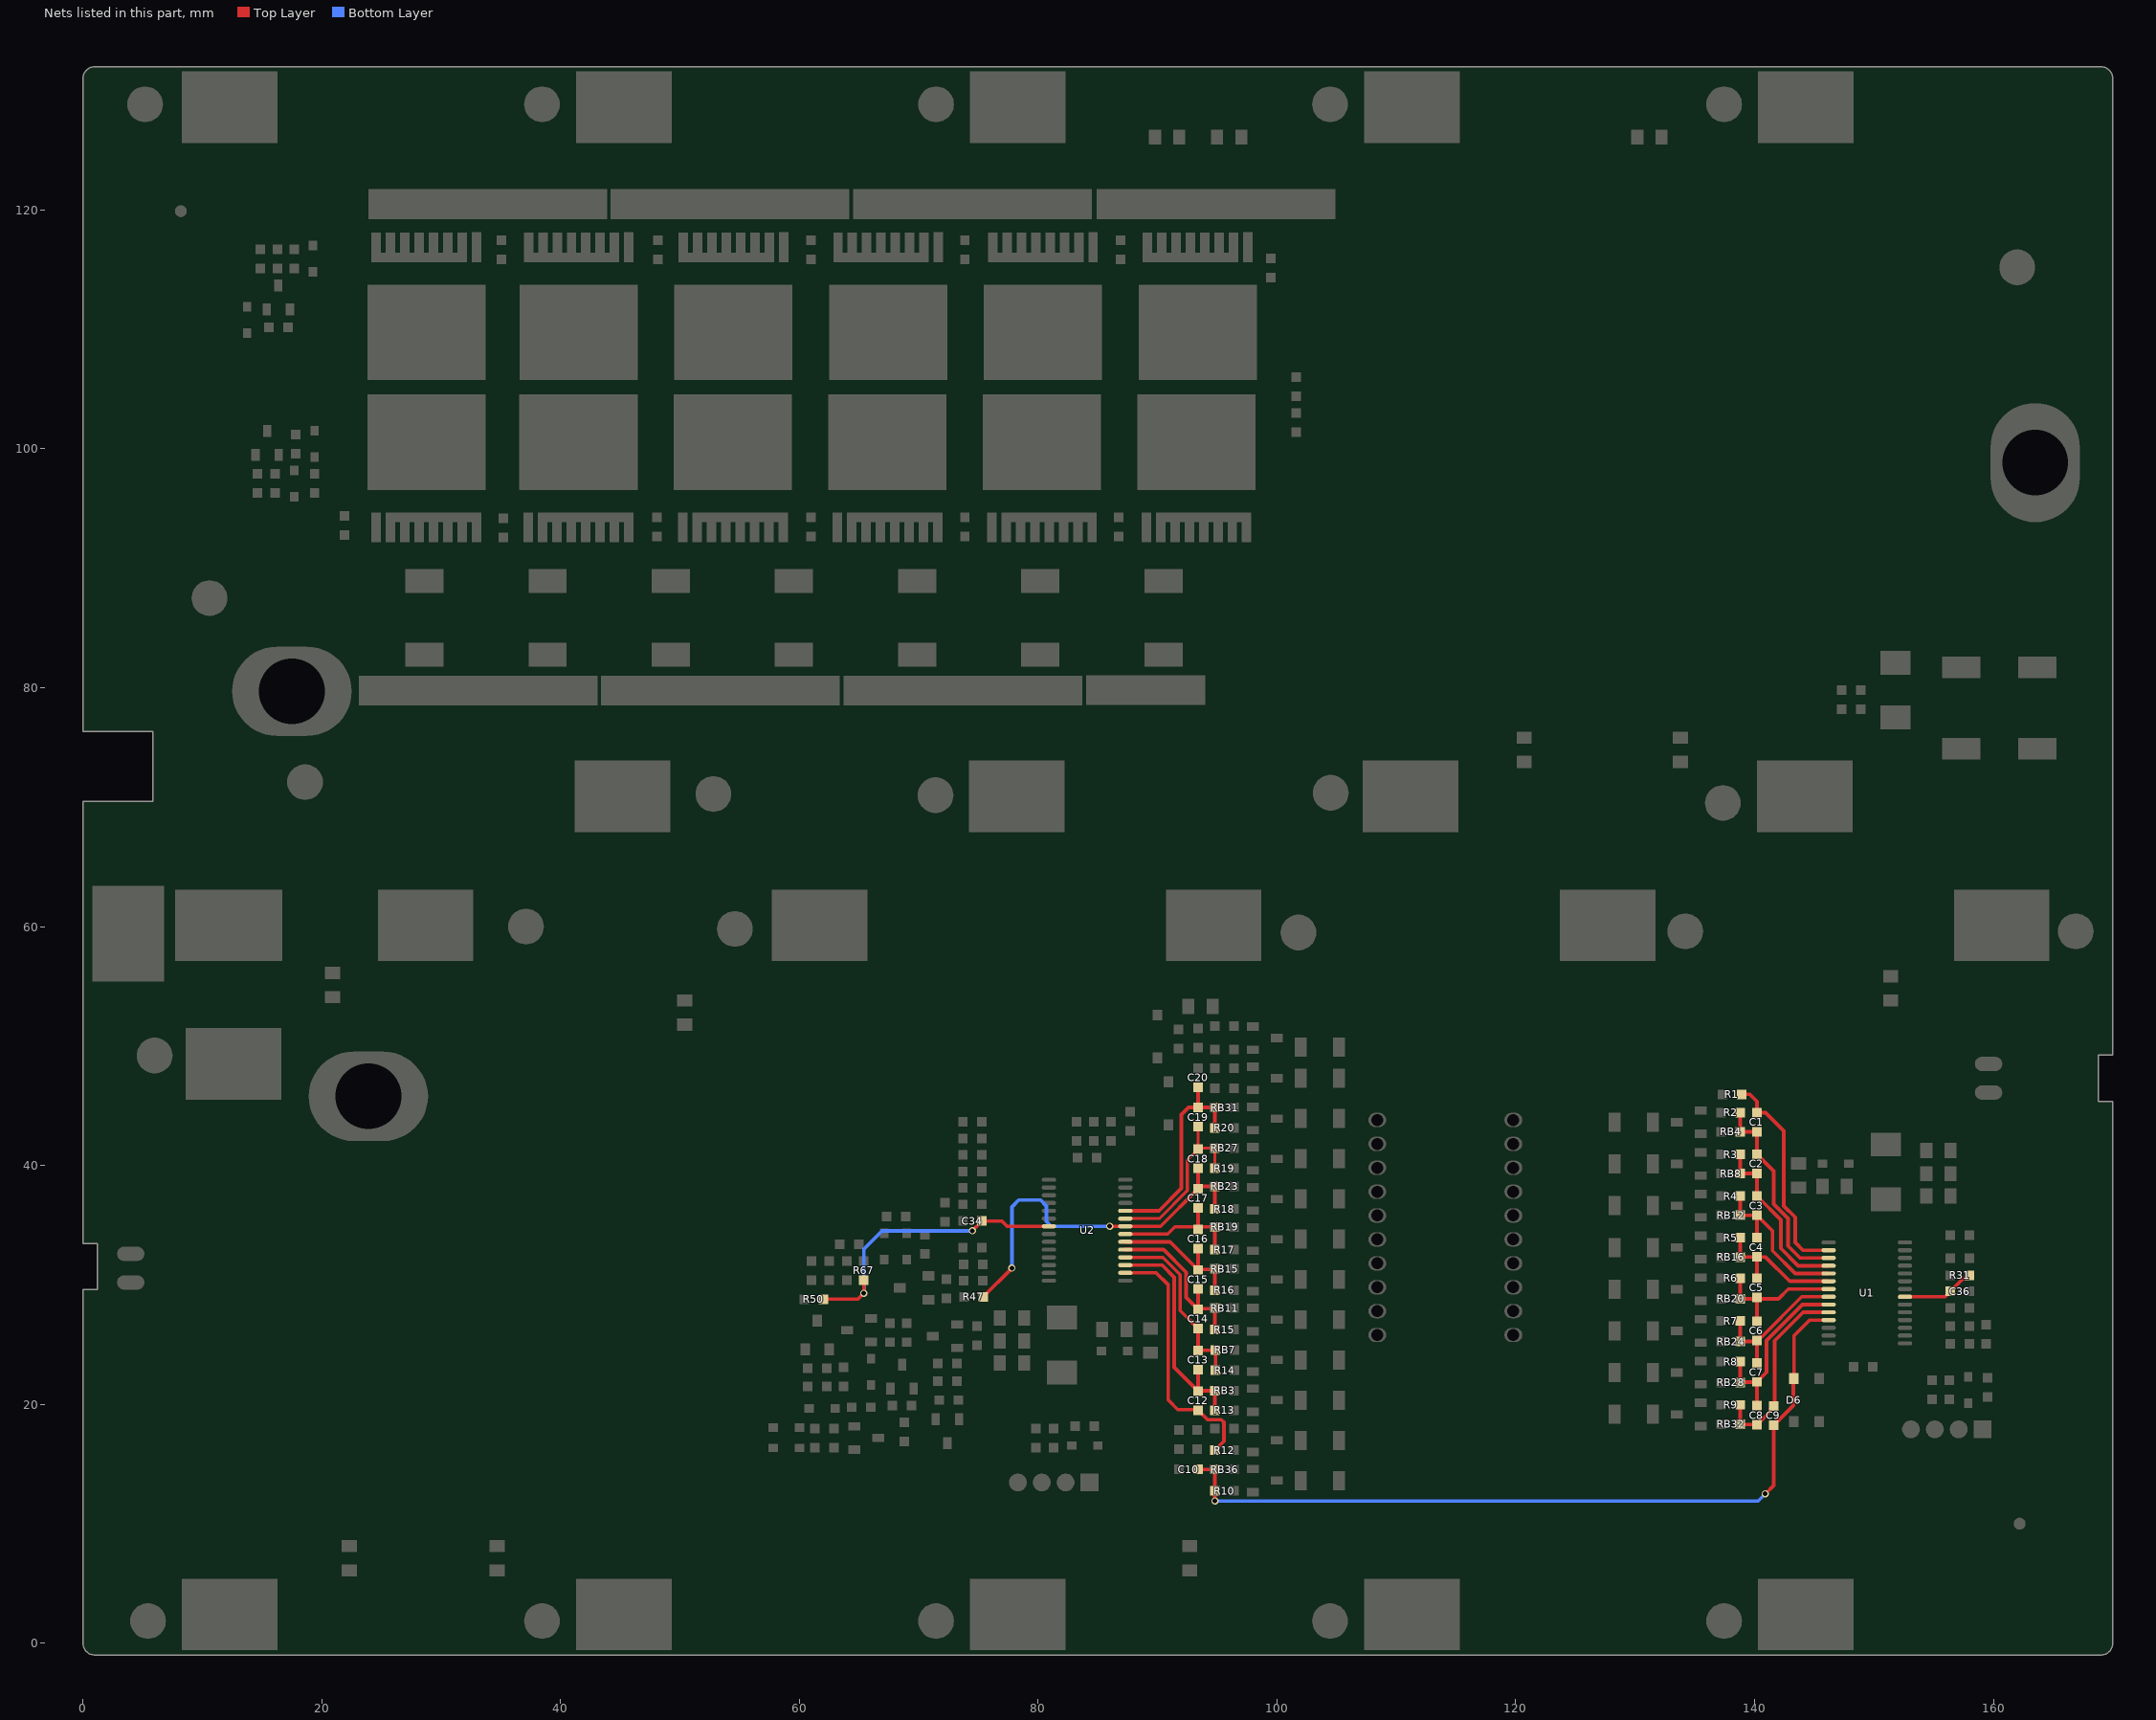
[diagram p0: the nets of this part, all layers, seen from the top]
# Altium PCB MISC82749.PcbDoc (part 4 of 4)
Units mm, origin at the board's own origin, x right, y up, seen from the top; angles counter-clockwise.
Board outline 170 x 133 mm, 2 copper layers (Top Layer, Bottom Layer); 262 components, 170 nets, 783 pads, 1052 vias.

## Via types
v1: diameter 0.7, hole 0.5, Top Layer to Bottom Layer, tented both sides, 953 vias
v2: diameter 0.6, hole 0.4, Top Layer to Bottom Layer, tented both sides, 99 vias

## Nets (pads, with @x,y where several pads share a name; then routed paths per layer and width w, separated by ;. In a path a pad name is that pad's centre, name@x,y a point inside that pad or via, vN(x,y) a via of type N, cw(c..) or ccw(c..) an arc to the next point about the centre after c; other vN are vias at no path point) (continued)
"VC1 S": C9.1 C10.2 D6.1 R10.2 RB36.2 U1.11 | length 68.1
  Top Layer w0.3: C10.2@93.4,14.55 93.45,14.5 93.5,14.55 RB36.2@94.8,14.55 v2(94.8,11.9) ; v2(140.9,12.5) 141.6,13.2 C9.1@141.6,18.25 143.25,19.9 143.25,22.1 D6.1@143.3,22.15 143.3,25.75 144.6,27.05 U1.11@146.2,27.05
  Bottom Layer w0.3: v2(94.8,11.9) 140.3,11.9 v2(140.9,12.5)
"VC2 M": C19.1 C20.2 R20.2 RB31.2 U2.10 | length 18.1
  Top Layer w0.3: U2.10@87.3,36.2 90.125,36.2 92,38.075 92,44.25 92.6,44.85 C19.1@93.4,44.85 ; C20.2@93.4,46.55 C19.1@93.4,44.85 ; R20.2@94.8,43.15 RB31.2@94.8,44.85 C19.1@93.4,44.85
"VC2 S": C8.1 C9.2 R9.2 RB32.2 U1.10 | length 16.2
  Top Layer w0.3: R9.2@138.8,19.882 RB32.2@138.8,18.332 138.825,18.307 140.175,18.307 C8.1@140.2,18.282 141.35,19.432 141.35,19.6 C9.2@141.6,19.85 ; C9.2@141.684,19.766 141.684,25.32 144.064,27.7 U1.10@146.2,27.7
"VC3 M": C18.1 C19.2 R19.2 RB27.2 U2.9 | length 15
  Top Layer w0.254: U2.9@87.3,35.55 90.15,35.55 92.5,37.9 92.5,40.45 C18.1@93.4,41.35 C18.1@93.4,41.45 ; C19.2@93.4,43.25 C18.1@93.4,41.45 ; R19.2@94.8,39.75 RB27.2@94.8,41.45 C18.1@93.4,41.45
"VC3 S": C7.1 C8.2 R8.2 RB28.2 U1.9 | length 15.4
  Top Layer w0.3: R8.2@138.8,23.573 RB28.2@138.8,21.83 138.821,21.852 140.179,21.852 C7.1@140.2,21.873 ; C8.2@140.2,19.883 C7.1@140.2,21.873 ; U1.9@146.2,28.35 144.007,28.35 141,25.343 141,22.673 C7.1@140.2,21.873
"VC4 M": C17.1 C18.2 R18.2 R47.2 RB23.2 U2.8 | length 32.1
  Top Layer w0.3: R47.2@75.4,29 v2(77.8,31.4) ; v2(86,34.9) U2.8@87.3,34.9 90.25,34.9 C17.1@93.4,38.05 ; C18.2@93.4,39.75 93.4,38.25 RB23.2@94.8,38.25 R18.2@94.8,36.35
  Bottom Layer w0.3: v2(77.8,31.4) 77.8,36.52 78.38,37.1 80.2,37.1 80.7,36.6 80.7,35.3 81.1,34.9 v2(86,34.9)
"VC4 S": C6.1 C7.2 R7.2 RB24.2 U1.8 | length 12.6
  Top Layer w0.3: R7.2@138.8,26.964 RB24.2@138.8,25.25 C6.1@140.2,25.25 ; C7.2@140.2,23.473 C6.1@140.2,25.25 ; U1.8@146.2,29 143.95,29 140.55,25.6 140.45,25.6 C6.1@140.2,25.35 ; C6.1@140.2,25.25 C6.1@140.2,25.35 ; C6.1@140.2,25.25 C6.1@140.2,25.35
"VC5 M": C16.1 C17.2 R17.2 RB19.2 U2.7 | length 11.4
  Top Layer w0.3: U2.7@87.3,34.25 90.849,34.25 91.449,34.85 C16.1@93.4,34.85 ; C16.1@93.4,34.65 C16.1@93.4,34.85 ; C17.2@93.4,36.45 C16.1@93.4,34.85 ; R17.2@94.8,32.95 RB19.2@94.8,34.85 C16.1@93.4,34.85
"VC5 S": C5.1 C6.2 R6.2 RB20.2 U1.7 | length 11.5
  Top Layer w0.3: R6.2@138.8,30.555 RB20.2@138.8,28.826 C5.1@140.2,28.826 ; C6.2@140.2,26.95 C5.1@140.2,28.826 ; C5.1@140.2,28.955 C5.1@140.2,28.826 ; U1.7@146.2,29.65 142.818,29.65 141.994,28.826 C5.1@140.2,28.826
"VC6 M": C15.1 C16.2 R16.2 RB15.2 U2.6 | length 12.1
  Top Layer w0.3: U2.6@87.3,33.6 91.05,33.6 C15.1@93.4,31.25 ; C16.2@93.4,33.05 C15.1@93.4,31.25 ; R16.2@94.8,29.55 RB15.2@94.8,31.35 94.75,31.3 93.45,31.3 C15.1@93.4,31.25
"VC6 S": C4.1 C5.2 R5.2 RB16.2 U1.6 | length 11.7
  Top Layer w0.3: R5.2@138.8,33.945 RB16.2@138.8,32.324 C4.1@140.2,32.324 ; C5.2@140.2,30.555 C4.1@140.2,32.324 ; C4.1@140.2,32.345 C4.1@140.2,32.324 ; U1.6@146.2,30.3 142.95,30.3 140.926,32.324 C4.1@140.2,32.324
"VC7 M": C14.1 C15.2 R15.2 RB11.2 U2.5 | length 14.3
  Top Layer w0.3: U2.5@87.3,32.95 90.5,32.95 92.4,31.05 92.4,28.95 C14.1@93.4,27.95 ; C15.2@93.4,29.65 C14.1@93.4,27.95 ; R15.2@94.8,26.25 RB11.2@94.8,28.05 94.75,28 93.45,28 C14.1@93.4,27.95
"VC7 S": C3.1 C4.2 R4.2 RB12.2 U1.5 | length 13.9
  Top Layer w0.3: R4.2@138.8,37.436 RB12.2@138.8,35.822 C3.1@140.2,35.822 ; C4.2@140.2,33.945 C3.1@140.2,35.822 ; C3.1@140.2,35.836 C3.1@140.2,35.822 ; U1.5@146.2,30.95 143.4,30.95 141.5,32.85 141.5,34.522 140.45,35.572 140.45,35.586 140.214,35.822 C3.1@140.2,35.822
"VC8 M": C13.1 C14.2 R14.2 RB7.2 U2.4 | length 15.3
  Top Layer w0.3: U2.4@87.3,32.3 90.443,32.3 91.9,30.843 91.9,27.85 C14.2@93.4,26.35 C13.1@93.4,24.5 93.425,24.525 94.825,24.525 RB7.2@94.85,24.55 R14.2@94.85,22.85
"VC8 S": C2.1 C3.2 R3.2 RB8.2 U1.4 | length 14.6
  Top Layer w0.3: R3.2@138.8,40.927 RB8.2@138.8,39.32 138.804,39.323 140.196,39.323 C2.1@140.2,39.327 C3.2@140.2,37.436 ; C3.2@140.3,37.337 142.2,35.436 142.2,33.05 143.65,31.6 U1.4@146.2,31.6
"VC9 M": C12.1 C13.2 R13.2 RB3.2 U2.3 | length 19.8
  Top Layer w0.3: U2.3@87.3,31.65 90.386,31.65 91.4,30.636 91.4,23.1 C12.1@93.4,21.1 ; C13.2@93.4,22.9 C12.1@93.4,21.1 ; R13.2@94.8,19.5 RB3.2@94.8,21.15 94.775,21.125 93.425,21.125 C12.1@93.4,21.1
"VC9 S": C1.1 C2.2 R2.2 RB4.2 U1.3 | length 17.5
  Top Layer w0.3: R2.2@138.8,44.418 RB4.2@138.8,42.818 C1.1@140.2,42.818 C2.2@140.2,40.927 141.6,39.527 141.6,36.75 142.8,35.55 142.8,33.25 143.8,32.25 U1.3@146.2,32.25
"VC10 M": C12.2 R12.2 U2.2 | length 21.7
  Top Layer w0.3: U2.2@87.3,31 89.893,31 90.9,29.993 90.9,20.35 91.7,19.55 93.35,19.55 C12.2@93.4,19.5 94.2,18.7 95.345,18.7 95.55,18.495 95.55,16.9 R12.2@94.8,16.15
"VC10 S": C1.2 R1.2 U1.2 | length 18.2
  Top Layer w0.3: R1.2@138.9,45.95 139.6,45.95 140.2,45.35 C1.2@140.2,44.418 140.932,44.418 142.454,42.896 142.454,36.604 143.4,35.657 143.4,33.55 144.05,32.9 U1.2@146.2,32.9
VCC_M: C34.2 R50.2 R67.2 U2.21 | length 25.1
  Top Layer w0.3: R50.2@62,28.8 64.9,28.8 v2(65.4,29.3) R67.2@65.4,30.4 ; v2(74.49,34.52) 74.49,34.53 C34.2@75.3,35.34 76.96,35.34 77.4,34.9 U2.21@80.9,34.9
  Bottom Layer w0.3: v2(65.4,29.3) 65.4,33 66.92,34.52 v2(74.49,34.52)
VCC_S: C36.2 R31.1 U1.21 | length 6.1
  Top Layer w0.3: U1.21@152.6,29 155.95,29 157.5,30.55 157.75,30.55 R31.1@158,30.8
pads on no net: U1.1 U1.27 U2.1 U2.27

## Polygon pours and split planes (outlines as drawn)
NetR68_2 on Top Layer "NONET_L02_P-001" (solid, remove dead copper, pour order 188): 155.6,50.4 161.1,50.4 161.4,50.1 161.4,47.5 155.7,47.5 155.6,47.6
NetR67_1 on Top Layer "NONET_L02_P-001" (solid, remove dead copper, pour order 187): 155.6,47 155.6,44.2 161.1,44.2 161.1,47
P-/C- on Top Layer "NONET_L02_P-001" (solid, remove dead copper, pour order 121): 20.8,124 127.5,124 127.75,123.75 128.7,122.8 170,122.8 170,79 170.1,78.9 102.6,78.9 102.6,105.2 102.4,105.4 101.1,105.4 101.1,116.3 100.831,116.569 99.431,116.569 99.062,116.938 99.062,118.338 96.96,118.338 96.96,115.689 96.821,115.55 87.65,115.55 87.5,115.7 87.5,118.1 87.262,118.338 84,118.338 84,115.55 74.46,115.55 74.46,118.25 74.372,118.338 71.04,118.338 71.04,115.55 61.56,115.55 61.56,118.25 61.472,118.338 58.08,118.338 58.08,115.55 48.76,115.55 48.76,118.35 45.132,118.35 45.12,118.338 45.12,115.55 35.66,115.55 35.66,118.05 35.372,118.338 32.36,118.338 32.36,115.61 32.3,115.55 20.402,115.55 19.8,116.152 19.8,123
B4 on Top Layer "NONET_L02_P-001" (solid, remove dead copper, pour order 139): 86.65,67.55 89.5,70.4 89.5,74.6 68.3,74.6 68.2,74.5 68.2,70.1 70.75,67.55
B14 on Top Layer "NONET_L02_P-001" (solid, remove dead copper, pour order 138): 98.3,63.4 98.9,62.8 105.5,62.8 105.8,62.5 105.8,59.375 105.8,55.35 88,55.35 88,63.4
B13 on Top Layer "NONET_L02_P-001" (solid, remove dead copper, pour order 131): 100,7.15 126.15,7.15 126.9,6.4 126.9,-0.4 126.4,-0.9 109.4,-0.9 100,-0.9
B+ on Top Layer "NONET_L02_P-001" (solid, remove dead copper, pour order 179): 0.1,27.546 30.993,27.546 31.5,27.039 31.5,9.6 31,9.1 0.6,9.1 0.1,9.6
B17 on Top Layer "NONET_L02_P-001" (solid, remove dead copper, pour order 129): 61.15,7.15 61.5,6.8 61.5,-0.9 34,-0.9 34,7.15
B+ on Top Layer "NONET_L02_P-001" (solid, remove dead copper, pour order 178): 155.1,44.2 155.1,52.7 125.2,52.7 125.2,43.1 125.5,42.8 129.9,42.8 129.9,44.8 131.6,46.5 141.5,46.5 144.8,44.2
B10 on Top Layer "NONET_L02_P-001" (solid, remove dead copper, pour order 170): 162.1,15.2 161.5,14.6 153.7,14.6 153.5,14.8 153.5,20.75 153.15,21.1 144.227,21.1 143.607,20.48 143.607,19.752 141.957,18.102 141.957,8.743 142.3,8.4 169.9,8.4 170,8.5 170,35.6 170,57.4 162.1,57.4
GND on Top Layer "NONET_L02_P-001" (solid, remove dead copper, pour order 186): 85.7,51 85.4,51.3 74,51.3 72.2,49.5 72.2,45.4 72.3,45 85.1,45 85.7,45.6
B12 on Top Layer "NONET_L02_P-001" (solid, remove dead copper, pour order 141): 120.9,62.6 121.2,62.9 125.5,62.9 141.7,62.9 141.7,55.35 120.9,55.35
NetC33_1 on Top Layer "NONET_L02_P-001" (solid, remove dead copper, pour order 184): 9.2,34.9 9.1,35 0.4,35 0.25,34.85 0.25,31.7 9.2,31.7
GND on Top Layer "NONET_L02_P-001" (solid, remove dead copper, pour order 183): 0.3,31.3 9.3,31.3 9.3,29.55 9.3,28.3 9.2,28.2 0.5,28.2 0.3,28.4
GND on Top Layer "NONET_L02_P-001" (solid, remove dead copper, pour order 182): 68.6,40.4 68.9,40.7 68.9,49.3 67.7,50.5 54.7,50.5 36.1,50.384 36.1,40.4
B10 on Top Layer "NONET_L02_P-001" (solid, remove dead copper, pour order 177): 116.1,78.2 116.1,76.1 144.8,76.1 144.8,78.3 116.5,78.3
VBAT_S on Top Layer "NONET_L02_P-001" (solid, remove dead copper, pour order 168): 154.1,34.3 154.1,33.8 154.2,33.7 154.7,33.7 155.712,34.712 157.12,36.12 157.12,42.98 156.8,43.3 155.7,43.3 155.7,35.9
B10 on Top Layer "NONET_L02_P-001" (solid, remove dead copper, pour order 167): 155.05,36.45 155.05,36.15 153.7,34.8 147.6,34.8 147.2,35.2 147.2,39.1 152.2,39.1 153.225,40.125 155.075,40.125 155.1,40.1 155.1,36.5
NetD1_1 on Top Layer "NONET_L02_P-001" (solid, remove dead copper, pour order 166): 152.9,40.5 154.9,40.5 155.1,40.7 155.1,43.4 147.2,43.4 147.2,39.5 151.9,39.5
NetC23_2 on Top Layer "NONET_L02_P-001" (solid, remove dead copper, pour order 165): 142.875,39.15 142.875,37.125 143.6,36.4 146.2,36.4 146.2,40.8 146.1,40.9 145.2,40.9 144.8,40.5 144.8,39.425 144.475,39.1 143.1,39.1
B6 on Top Layer "NONET_L02_P-001" (solid, remove dead copper, pour order 140): 121.8,68.5 121.6,68.3 115.2,68.3 114.7,67.8 103.151,67.8 102.5,68.451 102.5,73.7 103.2,74.4 121.4,74.4 121.8,74
VBAT_M on Top Layer "NONET_L02_P-001" (solid, remove dead copper, pour order 164): 77.7,27.824 80.376,30.5 78.805,30.5 76.09,27.785 76.09,21.61 76.5,21.2 77.5,21.2 77.7,21.4
NetC24_2 on Top Layer "NONET_L02_P-001" (solid, remove dead copper, pour order 162): 88.3,25.1 88.7,25.5 90.1,25.5 90.2,25.6 90.2,27.016 90.235,27.051 86.8,27 86.8,23.6 88.3,23.6
GND on Top Layer "NONET_L02_P-001" (solid, remove dead copper, pour order 161): 86.2,25.7 86.2,27.2 86.3,27.3 90.2,27.3 90.2,29.2 89.702,29.698 86.102,29.698 85.5,30.3 85.5,38.4 82.8,38.4 82,37.6 82,29.8 81.6,29.4 79.7,29.4 78.3,28 78.3,24.6 78.4,24.5 80.3,24.5 81.3,25.5 86,25.5
NetD2_1 on Top Layer "NONET_L02_P-001" (solid, remove dead copper, pour order 160): 78.4,24.2 78.4,22.2 79.5,21.1 85.7,21.1 85.9,21.3 85.9,24.9 81.7,24.9 81,24.2 78.7,24.2
GND on Top Layer "NONET_L02_P-001" (solid, remove dead copper, pour order 101): 95.1,75.9 40.6,75.9 38.8,74.1 38.8,67.9 5.85,67.9 5.85,76.35 0,76.35 0,114.5 0.5,115 11.2,115 11.8,114.4 11.8,93 14.9,89.9 23.8,89.9 24.1,89.6 24.1,85.6 26.1,83.6 95.1,83.6 95.9,82.8 95.9,76.7
NetC45_2 on Top Layer "NONET_L02_P-001" (solid, remove dead copper, pour order 117): 98.3,88 102,88 102,94.1 101.5,94.6 89.92,94.6 89.91,94.61 89.91,92.06 89.68,91.83 86.17,91.83 85.95,92.05 85.95,94.12 85.46,94.61 76.97,94.61 76.97,92.15 76.732,91.912 73.288,91.912 73.05,92.15 73.05,94.35 72.7,94.7 64.12,94.7 64.03,94.61 64.03,92.08 63.8,91.85 60.55,91.85 60.35,92.05 60.35,94.55 60.2,94.7 51.18,94.7 51.09,94.61 51.09,91.94 50.85,91.7 47.6,91.7 47.15,92.15 47.15,94.65 47,94.8 38.34,94.8 38.15,94.61 38.15,91.9 37.95,91.7 34.6,91.7 34.35,91.95 34.35,94.15 33.89,94.61 25.21,94.61 25.21,88.19 25.4,88
B+ on Top Layer "NONET_L02_P-001" (solid, remove dead copper, pour order 134): 31.6,36.5 2.7,36.5 0.9,38.3 0.9,63.55 19.3,63.55 19.3,53.9 19.7,53.5 31.4,53.5 31.6,53.3
B9 on Top Layer "NONET_L02_P-001" (solid, remove dead copper, pour order 127): 131.7,131.998 131.7,125.2 170,125.2 170,132.303
B+ on Top Layer "NONET_L02_P-001" (solid, remove dead copper, pour order 144): 150.8,77.7 170.1,77.7 170.1,68.35 150.8,68.35
B8 on Top Layer "NONET_L02_P-001" (solid, remove dead copper, pour order 143): 129.7,74.4 149.2,74.4 149.2,68 129.7,68
B10 on Top Layer "NONET_L02_P-001" (solid, remove dead copper, pour order 142): 147.8,63 169.5,63 169.7,62.8 169.7,55.25 147.8,55.25
B16 on Top Layer "NONET_L02_P-001" (solid, remove dead copper, pour order 137): 49.4,63 52.1,63 52.4,63.3 68.5,63.3 68.5,53.3 49.4,53.3
B2 on Top Layer "NONET_L02_P-001" (solid, remove dead copper, pour order 136): 61.1,68.2 61,68.1 56,68.1 55.55,67.65 40.1,67.65 40.1,73.7 40.9,74.5 61.1,74.5
B18 on Top Layer "NONET_L02_P-001" (solid, remove dead copper, pour order 135): 34.8,63.5 35.3,63 44.4,63 44.4,55.45 20,55.45 20,63.5
B11 on Top Layer "NONET_L02_P-001" (solid, remove dead copper, pour order 133): 169.7,7.15 170.2,6.45 170.2,-0.45 169.75,-0.9 133,-0.9 133,7.15
B15 on Top Layer "NONET_L02_P-001" (solid, remove dead copper, pour order 130): 93.65,7.15 94.3,6.5 94.3,-0.5 93.9,-0.9 76.4,-0.9 67,-0.9 67,7.15
B19 on Top Layer "NONET_L02_P-001" (solid, remove dead copper, pour order 128): 0,6.6 24.1,6.6 24.1,-0.65 23.75,-1 0,-1
B7 on Top Layer "NONET_L02_P-001" (solid, remove dead copper, pour order 126): 96.4,131.979 96.4,125.2 124.7,125.2 124.7,132.205
B5 on Top Layer "NONET_L02_P-001" (solid, remove dead copper, pour order 125): 61.9,131.967 61.9,125.2 90.6,125.2 90.6,132.196
B3 on Top Layer "NONET_L02_P-001" (solid, remove dead copper, pour order 124): 33,132 33,125.2 59.7,125.2 59.7,132.213
B1 on Top Layer "NONET_L02_P-001" (solid, remove dead copper, pour order 123): 30.5,125.4 30.5,132.191 24,132.191 0,132 0,125 18.6,125 19,125.4
MSO_D- on Top Layer "NONET_L02_P-001" (solid, remove dead copper, pour order 106): 22.105,95.995 20.3,97.8 20.3,113.8 21.093,114.593 23.143,114.593 23.15,114.6 98.25,114.6 98.95,113.9 98.95,113.85 100.6,113.85 100.6,95.995
GND on Bottom Layer "NONET_L02_P-001" (solid, remove dead copper, pour order 180): 63.043,29.857 63.043,32.057 62.8,32.3 62,32.3 61.6,32.7 61.6,36.1 62.995,37.495 80.705,37.495 81.2,37 81.2,35.7 81.5,35.4 84.05,35.4 86.4,35.4 86.6,35.2 86.6,34.3 86.4,34.1 80,34.1 79.3,33.4 79.3,22.7 81.2,20.8 87.6,20.8 87.9,21.1 87.9,23.5 88.5,24.1 102.9,24.1 103.3,24.5 103.2,24.6 103.2,43.4 57,43.4 56.869,43.269 35.769,43.269 34.8,42.3 34.8,15.6 37.1,13.3 76.9,13.3 77.6,14 77.6,15.5 77.4,15.7 67.4,15.7 63.1,20 63.1,29.8
B+ on Bottom Layer "NONET_L02_P-001" (solid, remove dead copper, pour order 172): 155.3,11.5 158.6,14.8 158.6,37.2 150.8,45 150.85,76.2 150.95,76.3 170.3,76.3 170.2,76.2 170.2,-0.45 169.75,-0.9 0.5,-0.9 -0.1,-0.3 -0.1,61.7 31.6,61.7 31.6,15.6 35.8,11.5
GND on Bottom Layer "NONET_L02_P-001" (solid, remove dead copper, pour order 181): 56,62 63.5,62 64.3,61.2 64.3,55.8 65.4,54.7 77.9,54.7 79.5,53.1 79.5,46 78.6,45.1 39.7,45.1 38.6,46.2 38.6,60 40.3,61.7 51.075,61.7 51.2,61.825 51.2,69.1 51.5,69.4 55.7,69.4 55.7,62.3
GND on Bottom Layer "NONET_L02_P-001" (solid, remove dead copper, pour order 185): 105.4,48.3 105.4,47.4 105.2,47.2 83.2,47.2 82.8,47.6 82.8,50.3 82.9,50.4 88,50.4 88.9,51.3 88.9,56.5 90.523,58.123 93.436,58.123 93.6,58.2 105.1,58.2 105.4,57.9
B10 on Bottom Layer "NONET_L02_P-001" (solid, remove dead copper, pour order 171): 130.55,61.85 130.9,62.2 133.6,62.2 133.8,62.4 133.8,68.3 133.6,68.5 122.2,68.5 121.8,68.9 121.8,78 122.2,78.4 130.55,78.4 145.4,78.4 145.5,78.3 145.5,69.2 144.8,68.5 138.4,68.5 138.1,68.2 138.1,62.5 138.6,62 148,62 148.9,61.1 148.9,48.6 148.9,44.5 155.1,38.3 155.1,34.6 154.706,34.206 151.806,34.206 147.7,30.1 147.7,19.5 147.5,19.3 136.2,19.3 135.8,19.7 135.8,21.7 130.5,27 130.5,59.9 130.55,59.95
P-/C- on Bottom Layer "NONET_L02_P-001" (solid, remove dead copper, pour order 175): 0.4,115.8 0,116.2 0,126.7 0.307,127.007 14.2,127.007 114.198,126.504 115.5,125.197 115.5,115.8
P-/C- on Bottom Layer "NONET_L02_P-001" (solid, remove dead copper, pour order 176): 127.6,124.9 128.2,125.5 128.2,128.5 128.9,129.2 129.7,129.2 147.3,129.2 169.6,129.2 170.2,128.6 170.2,79.8 169.3,78.9 124.1,78.9 122.8,80.2 122.8,124.5 123.2,124.9
MSO_D- on Bottom Layer "NONET_L02_P-001" (solid, remove dead copper, pour order 174): 14.2,114.7 14.5,115 115.5,115 115.5,96.5 14.4,96.5 14.2,96.7
NetC45_2 on Bottom Layer "NONET_L02_P-001" (solid, remove dead copper, pour order 173): 114.8,88.5 114.4,88.1 15.3,88.1 14.4,89 14.4,95.7 14.7,96 17.6,96 102.2,95.8 114.8,95.8
GND on Bottom Layer "NONET_L02_P-001" (solid, remove dead copper, pour order 114): 100.5,68.5 101.6,69.6 101.6,85.5 100.6,86.5 13.5,86.5 11.4,88.6 11.4,107.15 11.4,114.8 11.2,115 0.5,115 0,114.5 0,68.5

## Keep-outs
Keep-Out Layer:
  lines w0.1: 0,0 ccw(c1,0) 1,-1 169,-1 ccw(c169,0) 170,0 170,45.375 168.8,45.375 168.8,49.225 170,49.225 170,131 ccw(c169,131) 169,132 1,132 ccw(c1,131) 0,131 0,76.35 5.85,76.35 5.85,70.5 0,70.5 0,39.375 0,33.45 1.2,33.45 1.2,29.6 0,29.6 0,0 ; 7.2,63.5 7.2,67.5 17.2,67.5 17.2,63.5 7.2,63.5 ; 23.7,63.5 23.7,67.5 33.7,67.5 33.7,63.5 23.7,63.5 ; 40.2,63.5 40.2,67.5 50.2,67.5 50.2,63.5 40.2,63.5 ; 56.7,63.5 56.7,67.5 66.7,67.5 66.7,63.5 56.7,63.5 ; 73.2,63.5 73.2,67.5 83.2,67.5 83.2,63.5 73.2,63.5 ; 89.7,63.5 89.7,67.5 99.7,67.5 99.7,63.5 89.7,63.5 ; 106.2,63.5 106.2,67.5 116.2,67.5 116.2,63.5 106.2,63.5 ; 122.7,63.5 122.7,67.5 132.7,67.5 132.7,63.5 122.7,63.5 ; 139.2,63.5 139.2,67.5 149.2,67.5 149.2,63.5 139.2,63.5 ; 155.7,63.5 165.7,63.5 165.7,67.5 155.7,67.5 155.7,63.5

## Other copper
Top Layer:
  pour cut-out: 6.95,63.25 17.45,63.25 17.45,67.75 6.95,67.75
  pour cut-out: 23.45,63.25 33.95,63.25 33.95,67.75 23.45,67.75
  pour cut-out: 39.95,63.25 50.45,63.25 50.45,67.75 39.95,67.75
  pour cut-out: 56.45,63.25 66.95,63.25 66.95,67.75 56.45,67.75
  pour cut-out: 72.95,63.25 83.45,63.25 83.45,67.75 72.95,67.75
  pour cut-out: 89.45,63.25 99.95,63.25 99.95,67.75 89.45,67.75
  pour cut-out: 105.95,63.25 116.45,63.25 116.45,67.75 105.95,67.75
  pour cut-out: 122.45,63.25 132.95,63.25 132.95,67.75 122.45,67.75
  pour cut-out: 138.95,63.25 149.45,63.25 149.45,67.75 138.95,67.75
  pour cut-out: 155.4,63.15 166,63.15 166.05,63.2 166.05,67.8 166,67.85 155.4,67.85 155.35,67.8
Bottom Layer:
  pour cut-out: 6.2,62.5 6.2,68.5 18.2,68.5 18.2,62.5
  pour cut-out: 22.7,62.5 22.7,68.5 34.7,68.5 34.7,62.5
  pour cut-out: 39.2,62.5 39.2,68.5 51.2,68.5 51.2,62.5
  pour cut-out: 55.7,62.5 55.7,68.5 67.7,68.5 67.7,62.5
  pour cut-out: 72.2,62.5 72.2,68.5 84.2,68.5 84.2,62.5
  pour cut-out: 88.7,62.5 88.7,68.5 100.7,68.5 100.7,62.5
  pour cut-out: 105.2,62.5 105.2,68.5 117.2,68.5 117.2,62.5
  pour cut-out: 121.7,62.5 121.7,68.5 133.7,68.5 133.7,62.5
  pour cut-out: 138.2,62.5 138.2,68.5 150.2,68.5 150.2,62.5
  pour cut-out: 154.7,62.5 154.7,68.5 166.7,68.5 166.7,62.5

## Silkscreen, mask and mechanical layers (free items; w line width, h text height)
Mechanical 1:
  lines w0.1: -7.75,129 193.35,129 ; 0,65.5 170,65.5 ; 0,0 ccw(c1,0) 1,-1 169,-1 ccw(c169,0) 170,0 170,131 ccw(c169,131) 169,132 1,132 ccw(c1,131) 0,131 0,0
Mechanical 3:
  drawing of 235 lines, arcs and shapes, not listed
  text "B1" at 18.5,123.1 h6
  text "B7" at 111.162,121.283 h6
  text "B9" at 141.262,121.15 h6
  text "B3" at 49.05,120.767 h6
  text "B5" at 82.8,120.617 h6
  text "B1" at 3.95,116.35 h3
  text "B12" at 3.6,87.3 h3
  text "B8" at 137.762,76.15 h6
  text "B4" at 77.7,75.5 h6
  text "B6" at 109.4,75.417 h6
  text "B2" at 42.6,75.35 h6
  text "B10" at 157.162,51.85 h6
  text "B18" at 25,51.217 h6
  text "B14" at 97.1,51.2 h6
  text "B16" at 62,51.117 h6
  text "B12" at 128.8,51.05 h6
  text "B20" at 6.7,50.917 h6
  text "B13" at 3.75,36.033 h3
  text "B20" at 3.6,15.333 h3
  text "B13" at 106.65,8.867 h6
  text "B15" at 71.55,8.717 h6
  text "B11" at 138.85,8.4 h6
  text "B17" at 42.3,8.15 h6
  text "B19" at 7.2,8.067 h6